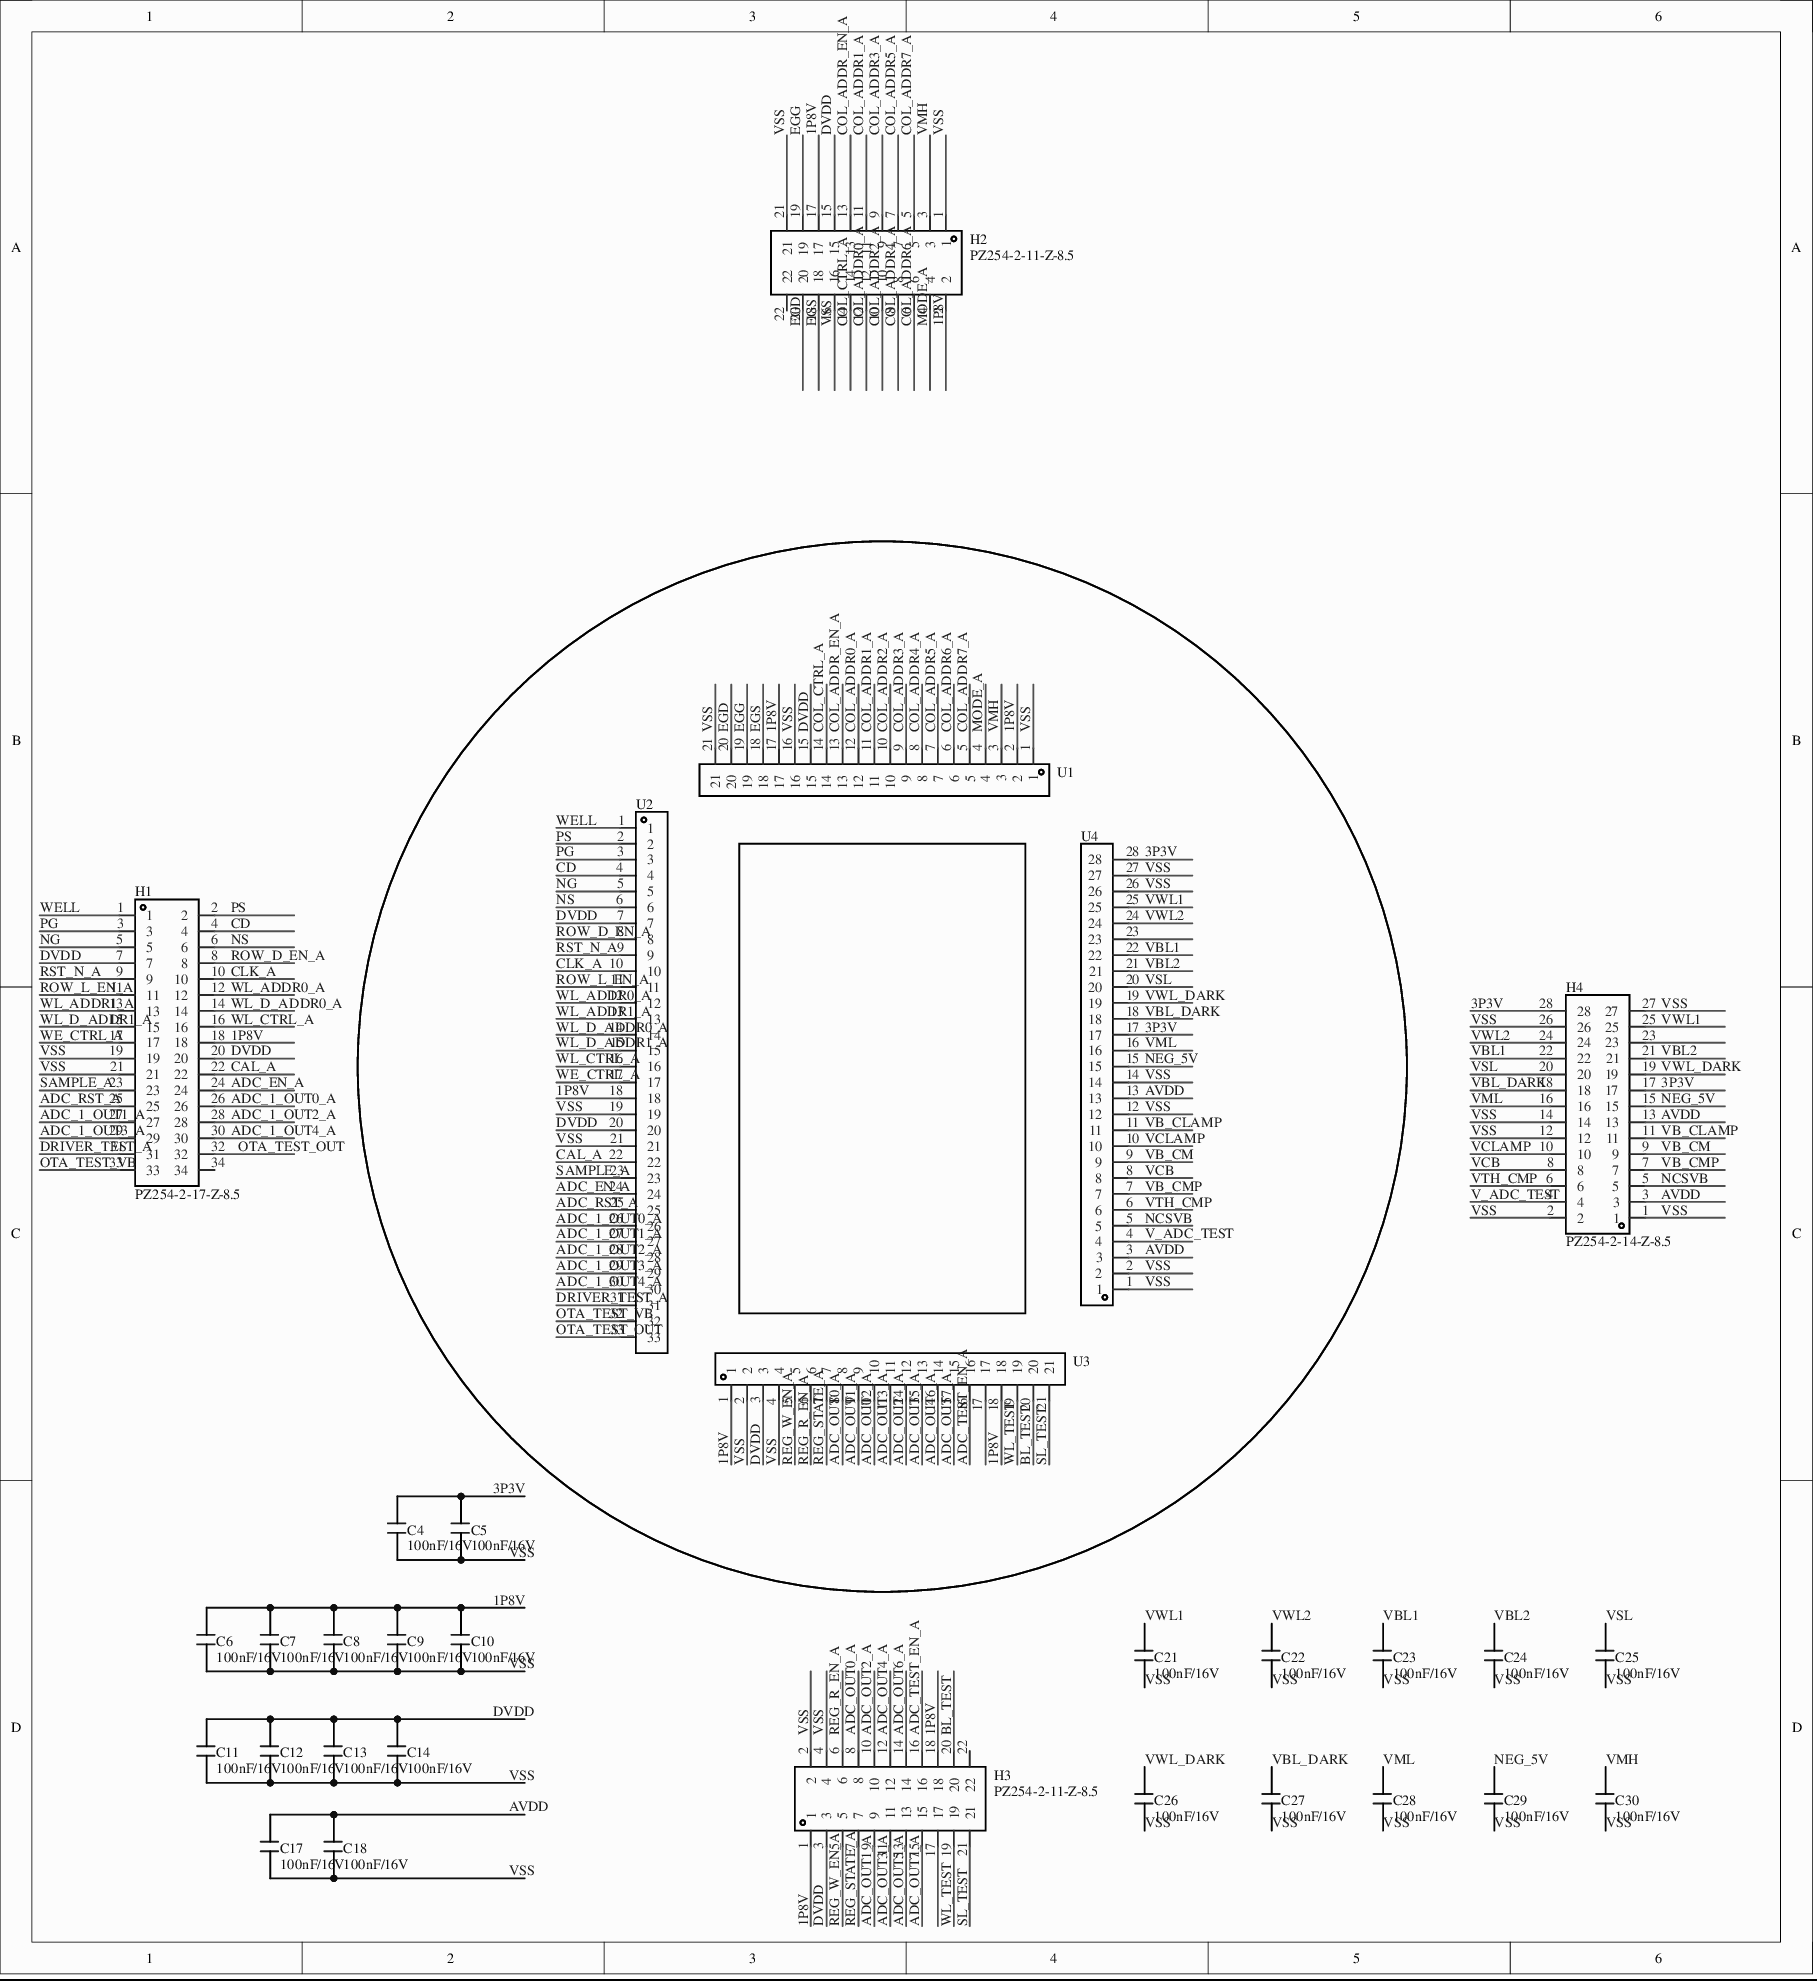
[diagram p0: MISC79019-2.schdoc]
# Altium project MISC79019-7.PrjPCB
1 sheet, 31 parts. Net scope: global (net labels, ports and power ports of the same name join across sheets).
Board file: MISC79019.PcbDoc

## Sheet MISC79019-2.schdoc
size 289 x 314 mm

### Parts
C4  100nF/16V  [0603C]
C5  100nF/16V  [0603C]
C6  100nF/16V  [0603C]
C7  100nF/16V  [0603C]
C8  100nF/16V  [0603C]
C9  100nF/16V  [0603C]
C10  100nF/16V  [0603C]
C11  100nF/16V  [0603C]
C12  100nF/16V  [0603C]
C13  100nF/16V  [0603C]
C14  100nF/16V  [0603C]
C17  100nF/16V  [0603C]
C18  100nF/16V  [0603C]
C21  100nF/16V  [0603C]
C22  100nF/16V  [0603C]
C23  100nF/16V  [0603C]
C24  100nF/16V  [0603C]
C25  100nF/16V  [0603C]
C26  100nF/16V  [0603C]
C27  100nF/16V  [0603C]
C28  100nF/16V  [0603C]
C29  100nF/16V  [0603C]
C30  100nF/16V  [0603C]
H1  PZ254-2-17-Z-8.5  [HDR-TH_34P-P2.54-V-M-R2-C17-S2.54]
H2  PZ254-2-11-Z-8.5  [HDR-TH_22P-P2.54-V-M-R2-C11-S2.54]
H3  PZ254-2-11-Z-8.5  [HDR-TH_22P-P2.54-V-M-R2-C11-S2.54]
H4  PZ254-2-14-Z-8.5  [HDR-TH_28P-P2.54-V-M-R2-C14-S2.54]
U1  X6511WVS-21H-C60D48R2  [JSZ21]  (value not drawn)
U2  X6511WVS-33H-C60D48R2  [JSZ33]  (value not drawn)
U3  X6511WVS-21H-C60D48R2  [JSZ21]  (value not drawn)
U4  X6511WVS-28H-C60D48R1  [JSZ28]  (value not drawn)

### Nets
1P8V: C6.1 C7.1 C8.1 C9.1 C10.1 H1.18 H2.2 H2.17 H3.1 H3.18 U1.2 U1.17 U2.18 U3.1 U3.18
3P3V: C4.1 C5.1 H4.17 H4.28 U4.17 U4.28
ADC_1_OUT0_A: H1.26 U2.26
ADC_1_OUT1_A: H1.27 U2.27
ADC_1_OUT2_A: H1.28 U2.28
ADC_1_OUT3_A: H1.29 U2.29
ADC_1_OUT4_A: H1.30 U2.30
ADC_EN_A: H1.24 U2.24
ADC_OUT0_A: H3.8 U3.8
ADC_OUT1_A: H3.9 U3.9
ADC_OUT2_A: H3.10 U3.10
ADC_OUT3_A: H3.11 U3.11
ADC_OUT4_A: H3.12 U3.12
ADC_OUT5_A: H3.13 U3.13
ADC_OUT6_A: H3.14 U3.14
ADC_OUT7_A: H3.15 U3.15
ADC_RST_A: H1.25 U2.25
ADC_TEST_EN_A: H3.16 U3.16
AVDD: C17.1 C18.1 H4.3 H4.13 U4.3 U4.13
BL_TEST: H3.20 U3.20
CAL_A: H1.22 U2.22
CD: H1.4 U2.4
CLK_A: H1.10 U2.10
COL_ADDR0_A: H2.12 U1.12
COL_ADDR1_A: H2.11 U1.11
COL_ADDR2_A: H2.10 U1.10
COL_ADDR3_A: H2.9 U1.9
COL_ADDR4_A: H2.8 U1.8
COL_ADDR5_A: H2.7 U1.7
COL_ADDR6_A: H2.6 U1.6
COL_ADDR7_A: H2.5 U1.5
COL_ADDR_EN_A: H2.13 U1.13
COL_CTRL_A: H2.14 U1.14
DRIVER_TEST_A: H1.31 U2.31
DVDD: C11.1 C12.1 C13.1 C14.1 H1.7 H1.20 H2.15 H3.3 U1.15 U2.7 U2.20 U3.3
EGD: H2.20 U1.20
EGG: H2.19 U1.19
EGS: H2.18 U1.18
MODE_A: H2.4 U1.4
NCSVB: H4.5 U4.5
NEG_5V: C29.1 H4.15 U4.15
NG: H1.5 U2.5
NS: H1.6 U2.6
OTA_TEST_OUT: H1.32 U2.33
OTA_TEST_VB: H1.33 U2.32
PG: H1.3 U2.3
PS: H1.2 U2.2
REG_R_EN_A: H3.6 U3.6
REG_STATE_A: H3.7 U3.7
REG_W_EN_A: H3.5 U3.5
ROW_D_EN_A: H1.8 U2.8
ROW_L_EN_A: H1.11 U2.11
RST_N_A: H1.9 U2.9
SAMPLE_A: H1.23 U2.23
SL_TEST: H3.21 U3.21
V_ADC_TEST: H4.4 U4.4
VB_CLAMP: H4.11 U4.11
VB_CM: H4.9 U4.9
VB_CMP: H4.7 U4.7
VBL1: C23.1 H4.22 U4.22
VBL2: C24.1 H4.21 U4.21
VBL_DARK: C27.1 H4.18 U4.18
VCB: H4.8 U4.8
VCLAMP: H4.10 U4.10
VMH: C30.1 H2.3 U1.3
VML: C28.1 H4.16 U4.16
VSL: C25.1 H4.20 U4.20
VSS: C4.2 C5.2 C6.2 C7.2 C8.2 C9.2 C10.2 C11.2 C12.2 C13.2 C14.2 C17.2 C18.2 C21.2 C22.2 C23.2 C24.2 C25.2 C26.2 C27.2 C28.2 C29.2 C30.2 H1.19 H1.21 H2.1 H2.16 H2.21 H3.2 H3.4 H4.1 H4.2 H4.12 H4.14 H4.26 H4.27 U1.1 U1.16 U1.21 U2.19 U2.21 U3.2 U3.4 U4.1 U4.2 U4.12 U4.14 U4.26 U4.27
VTH_CMP: H4.6 U4.6
VWL1: C21.1 H4.25 U4.25
VWL2: C22.1 H4.24 U4.24
VWL_DARK: C26.1 H4.19 U4.19
WE_CTRL_A: H1.17 U2.17
WELL: H1.1 U2.1
WL_ADDR0_A: H1.12 U2.12
WL_ADDR1_A: H1.13 U2.13
WL_CTRL_A: H1.16 U2.16
WL_D_ADDR0_A: H1.14 U2.14
WL_D_ADDR1_A: H1.15 U2.15
WL_TEST: H3.19 U3.19

Not connected (* = marked no-connect by the designer): H1 34; H2 22; H3 17 22; H4 23; U3 17; U4 23

### Library data of the parts
C4-C14 C17 C18 C21-C30 = CAP: component CAP componentdescr capacitor model
H1 = PZ254-2-17-Z-8.5: Add into BOM: yes; Pin Structure: 2x17P; Pitch: 2.54mm; Current Rating (Max): 3A; Name: PZ254-2-17-Z-8.5; Symbol: PZ254-2-17-Z-8.5; Device: PZ254-2-17-Z-8.5; Supplier Part: C2894978; Manufacturer Part: PZ254-2-17-Z-8.5; Datasheet: https://atta.szlcsc.com/upload/public/pdf/source/20230609/5BA09C8BEB9B31376F8BF6032FF67CAC.pdf; Supplier: LCSC; Convert to PCB: yes; Row Spacing: 2.54mm; Number of Pins: 34P; Voltage Rating (Max): -; Length of Mating Pin: 6mm; Insulation Height: 2.5mm; Length of End Connection Pin: 3mm
H2 H3 = PZ254-2-11-Z-8.5: Add into BOM: yes; Pin Structure: 2x11P; Pitch: 2.54mm; Current Rating (Max): 3A; Name: PZ254-2-11-Z-8.5; Symbol: PZ254-2-11-Z-8.5; Device: PZ254-2-11-Z-8.5; Supplier Part: C2894972; Manufacturer Part: PZ254-2-11-Z-8.5; Datasheet: https://atta.szlcsc.com/upload/public/pdf/source/20230609/5BA09C8BEB9B31376F8BF6032FF67CAC.pdf; Supplier: LCSC; Convert to PCB: yes; Row Spacing: 2.54mm; Number of Pins: 22P; Voltage Rating (Max): -; Length of Mating Pin: 6mm; Insulation Height: 2.5mm; Length of End Connection Pin: 3mm
H4 = PZ254-2-14-Z-8.5: Add into BOM: yes; Pin Structure: 2x14P; Pitch: 2.54mm; Current Rating (Max): 3A; Name: PZ254-2-14-Z-8.5; Symbol: PZ254-2-14-Z-8.5; Device: PZ254-2-14-Z-8.5; Supplier Part: C2894975; Manufacturer Part: PZ254-2-14-Z-8.5; Datasheet: https://atta.szlcsc.com/upload/public/pdf/source/20230609/5BA09C8BEB9B31376F8BF6032FF67CAC.pdf; Supplier: LCSC; Convert to PCB: yes; Row Spacing: 2.54mm; Number of Pins: 28P; Voltage Rating (Max): -; Length of Mating Pin: 6mm; Insulation Height: 2.5mm; Length of End Connection Pin: 3mm
U1 U3 = X6511WVS-21H-C60D48R2: Add into BOM: no; Pin Structure: 1x21P; Pitch: 2.54mm; Current Rating (Max): 3A; Voltage Rating (Max): 250V; Origin Footprint 2: HDR-SMD_21P-P2.54-V-M-LS4.8_R2; Name: X6511WVS-21H-C60D48R2; Symbol: X6511WVS-21H-C60D48R2; Device: X6511WVS-21H-C60D48R2; Supplier Part: C2883778; Manufacturer Part: X6511WVS-21H-C60D48R2; Datasheet: https://atta.szlcsc.com/upload/public/pdf/source/20200909/C780060_F941EB1B69F43B5D6329EAF74E2E27BB.pdf; Supplier: LCSC; Convert to PCB: no; Row Spacing: 2.54mm; Number of Pins: 21P; Length of Mating Pin: 6mm; Insulation Height: 2.5mm; Length of End Connection Pin: 4.8mm; Origin Footprint 1: HDR-SMD_21P-P2.54-V-M-LS4.8_R2; Design Item ID: X6511WVS-21H-C60D48R2
U2 = X6511WVS-33H-C60D48R2: Add into BOM: no; Pin Structure: 1x33P; Pitch: 2.54mm; Current Rating (Max): 3A; Voltage Rating (Max): 250V; Origin Footprint 2: HDR-SMD_33P-P2.54-V-M-LS4.8_R2; Symbol: X6511WVS-33H-C60D48R2; Device: X6511WVS-33H-C60D48R2; Supplier Part: C2883790; Manufacturer Part: X6511WVS-33H-C60D48R2; Supplier Footprint: SMD,P=2.54mm; Datasheet: https://atta.szlcsc.com/upload/public/pdf/source/20200909/C780060_F941EB1B69F43B5D6329EAF74E2E27BB.pdf; Supplier: LCSC; Convert to PCB: no; Row Spacing: 2.54mm; Number of Pins: 33P; Length of Mating Pin: 6mm; Insulation Height: 2.5mm; Length of End Connection Pin: 4.8mm; Origin Footprint 1: HDR-SMD_33P-P2.54-V-M-LS4.8_R2; Design Item ID: X6511WVS-33H-C60D48R2
U4 = X6511WVS-28H-C60D48R1: Add into BOM: no; Pin Structure: 1x28P; Pitch: 2.54mm; Current Rating (Max): 3A; Voltage Rating (Max): 250V; Origin Footprint 2: HDR-SMD_28P-P2.54_XKBINDUSTRIAL_X6511WVS-28H-C60D48R1; Name: X6511WVS-28H-C60D48R1; Symbol: X6511WVS-28H-C60D48R1; Device: X6511WVS-28H-C60D48R1; Supplier Part: C2883824; Manufacturer Part: X6511WVS-28H-C60D48R1; Datasheet: https://atta.szlcsc.com/upload/public/pdf/source/20200909/C780060_F941EB1B69F43B5D6329EAF74E2E27BB.pdf; Supplier: LCSC; Convert to PCB: no; Row Spacing: 2.54mm; Number of Pins: 28P; Length of Mating Pin: 6mm; Insulation Height: 2.5mm; Length of End Connection Pin: 4.8mm; Origin Footprint 3: HDR-SMD_28P-P2.54_XKBINDUSTRIAL_X6511WVS-28H-C60D48R1; Origin Footprint 1: HDR-SMD_28P-P2.54_XKBINDUSTRIAL_X6511WVS-28H-C60D48R1; Design Item ID: X6511WVS-28H-C60D48R1